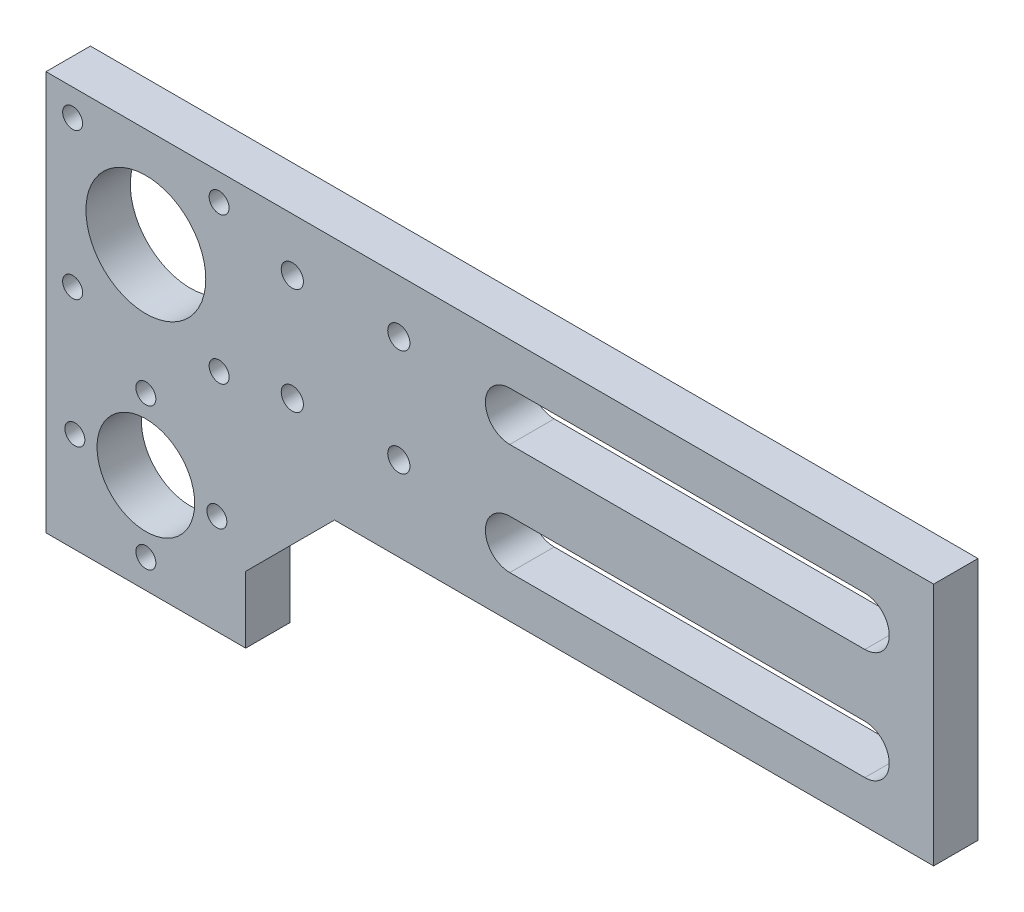
from build123d import *

# Parameters (mm, degrees)
SKETCH_2_R          = 11
SKETCH_2_R_2        = 13.5
SKETCH_2_R_3        = 2.25
EXTRUDE_1_DEPTH     = 10
CHAMFER_1_SIZE      = 20
CUT_EXTRUDE_1_REACH = 192.164
SKETCH_3_R          = 2.5


with BuildPart() as part:
    # 草图2 → 凸台-拉伸1 (new body)
    with BuildSketch(Plane.XY):
        Polygon((-22.5, 67.5), (177.5, 67.5), (177.5, 12.5), (22.5, 12.5), (22.5, -22.5), (-22.5, -22.5), align=None)
        Circle(SKETCH_2_R, mode=Mode.SUBTRACT)
        with Locations((0, 45)):
            Circle(SKETCH_2_R_2, mode=Mode.SUBTRACT)
        with Locations((-16.5, 61.5)):
            Circle(SKETCH_2_R_3, mode=Mode.SUBTRACT)
        with Locations(Location((16.5, 61.5, 0), (0, 0, 180))):
            Circle(SKETCH_2_R_3, mode=Mode.SUBTRACT)
        with Locations((16.5, 28.5)):
            Circle(SKETCH_2_R_3, mode=Mode.SUBTRACT)
        with Locations(Location((-16.5, 28.5, 0), (0, 0, 180))):
            Circle(SKETCH_2_R_3, mode=Mode.SUBTRACT)
        with Locations((0, 16)):
            Circle(SKETCH_2_R_3, mode=Mode.SUBTRACT)
        with Locations((16, 0)):
            Circle(SKETCH_2_R_3, mode=Mode.SUBTRACT)
        with Locations((0, -16)):
            Circle(SKETCH_2_R_3, mode=Mode.SUBTRACT)
        with Locations((-16, 0)):
            Circle(SKETCH_2_R_3, mode=Mode.SUBTRACT)
        with BuildLine():
            Line((162, 47), (82, 47))
            ThreePointArc((82, 47), (76.5, 52.5), (82, 58))
            Line((82, 58), (162, 58))
            ThreePointArc((162, 58), (167.5, 52.5), (162, 47))
        make_face(mode=Mode.SUBTRACT)
        with BuildLine():
            Line((162, 33), (82, 33))
            ThreePointArc((82, 33), (76.5, 27.5), (82, 22))
            Line((82, 22), (162, 22))
            ThreePointArc((162, 22), (167.5, 27.5), (162, 33))
        make_face(mode=Mode.SUBTRACT)
    extrude(amount=EXTRUDE_1_DEPTH)

    # 倒角1
    chamfer_1_edges = [part.edges().sort_by_distance(p)[0] for p in [
        (22.5, 12.5, 5),
    ]]
    chamfer(chamfer_1_edges, length=CHAMFER_1_SIZE)

    # 草图3 → 切除-拉伸1 (cut, up to next)
    with BuildSketch(Plane(origin=(0, 0, 0), x_dir=(-1, 0, 0), z_dir=(0, 0, -1)), mode=Mode.PRIVATE) as cut_extrude_1_sk1:
        with Locations((-57, 55.5)):
            Circle(SKETCH_3_R)
    cut_extrude_1_tool1 = extrude(cut_extrude_1_sk1.sketch, amount=-CUT_EXTRUDE_1_REACH, mode=Mode.PRIVATE) & part.part
    # 草图3 → 切除-拉伸1 (cut, up to next)
    with BuildSketch(Plane(origin=(0, 0, 0), x_dir=(-1, 0, 0), z_dir=(0, 0, -1)), mode=Mode.PRIVATE) as cut_extrude_1_sk2:
        with Locations((-33, 55.5)):
            Circle(SKETCH_3_R)
    cut_extrude_1_tool2 = extrude(cut_extrude_1_sk2.sketch, amount=-CUT_EXTRUDE_1_REACH, mode=Mode.PRIVATE) & part.part
    # 草图3 → 切除-拉伸1 (cut, up to next)
    with BuildSketch(Plane(origin=(0, 0, 0), x_dir=(-1, 0, 0), z_dir=(0, 0, -1)), mode=Mode.PRIVATE) as cut_extrude_1_sk3:
        with Locations((-33, 31.5)):
            Circle(SKETCH_3_R)
    cut_extrude_1_tool3 = extrude(cut_extrude_1_sk3.sketch, amount=-CUT_EXTRUDE_1_REACH, mode=Mode.PRIVATE) & part.part
    # 草图3 → 切除-拉伸1 (cut, up to next)
    with BuildSketch(Plane(origin=(0, 0, 0), x_dir=(-1, 0, 0), z_dir=(0, 0, -1)), mode=Mode.PRIVATE) as cut_extrude_1_sk4:
        with Locations((-57, 31.5)):
            Circle(SKETCH_3_R)
    cut_extrude_1_tool4 = extrude(cut_extrude_1_sk4.sketch, amount=-CUT_EXTRUDE_1_REACH, mode=Mode.PRIVATE) & part.part
    add(cut_extrude_1_tool1.solids().sort_by_distance((57, 55.5, 0))[0], mode=Mode.SUBTRACT)
    add(cut_extrude_1_tool2.solids().sort_by_distance((33, 55.5, 0))[0], mode=Mode.SUBTRACT)
    add(cut_extrude_1_tool3.solids().sort_by_distance((33, 31.5, 0))[0], mode=Mode.SUBTRACT)
    add(cut_extrude_1_tool4.solids().sort_by_distance((57, 31.5, 0))[0], mode=Mode.SUBTRACT)


solid = part.part
